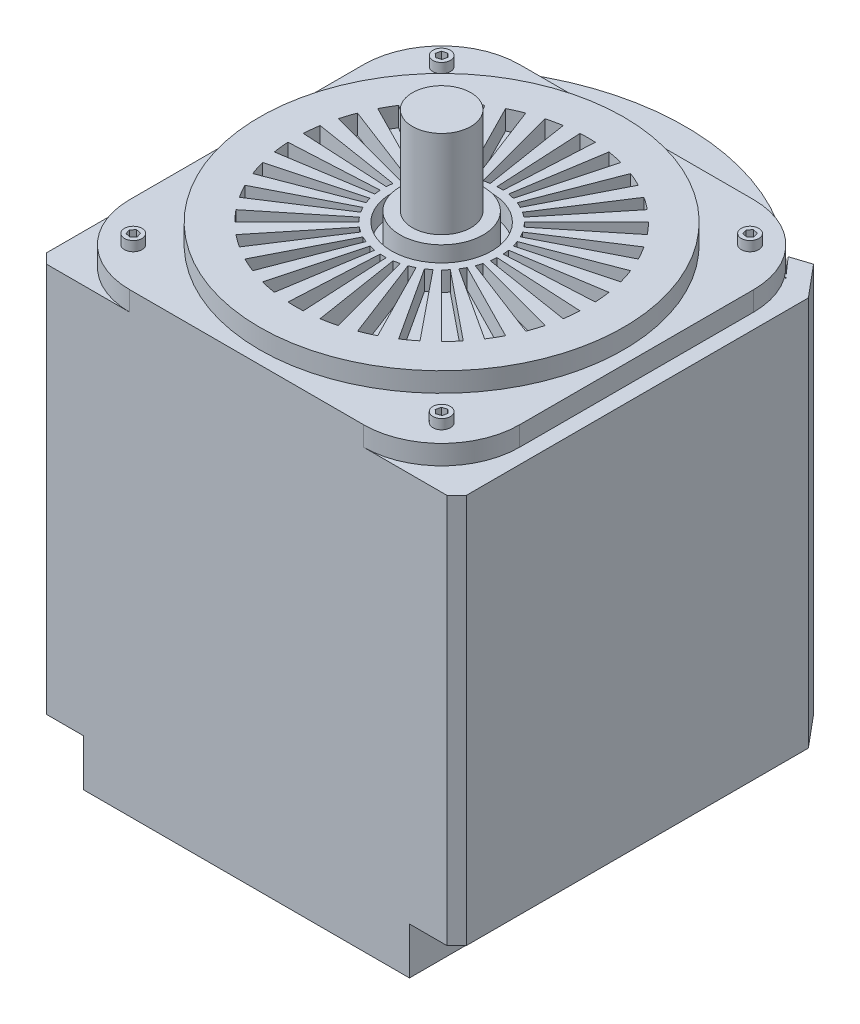
SolidWorks part; units mm, degrees
ref_plane "Front Plane" through (0, 0, 0) normal (0, 0, 1) x (1, 0, 0)
ref_plane "Top Plane" through (0, 0, 0) normal (0, 1, 0) x (1, 0, 0)
ref_plane "Right Plane" through (0, 0, 0) normal (1, 0, 0) x (0, 0, -1)
other "Configuration Table"
sketch "Sketch1" plane through (0, 0, 0) normal (0, 1, 0) x (1, 0, 0)
  line L0 (-1.5, 124.991) -> (-5.5544, 109.8597)
  line L1 (1.5, 124.991) -> (5.5544, 109.8597)
  line L2 (0, 125) -> (0, 0) construction
  line L3 (15.8617, 123.9895) -> (9.7465, 109.5674)
  line L4 (18.8327, 123.5732) -> (20.7479, 108.0256)
  line L5 (32.9165, 120.5882) -> (24.8588, 107.1543)
  line L6 (35.8009, 119.7635) -> (35.5397, 104.1006)
  line L7 (49.3341, 114.8527) -> (39.4899, 102.6672)
  line L8 (52.0761, 113.6357) -> (49.6436, 98.1606)
  line L9 (64.7968, 106.8942) -> (53.3567, 96.1928)
  line L10 (67.3434, 105.3084) -> (62.7867, 90.3207)
  line L11 (79.0053, 96.8667) -> (66.1907, 87.8566)
  line L12 (81.3072, 94.9428) -> (74.7145, 80.7326)
  line L13 (91.6846, 84.9643) -> (77.7436, 77.8199)
  line L15 (0, 0) -> (5.5544, 109.8597) construction
  line L16 (0, 0) -> (20.7479, 108.0256) construction
  line L17 (-15.91, 123.9834) -> (-9.7891, 109.5636)
  line L18 (-18.8808, 123.5658) -> (-20.7899, 108.0175)
  line L19 (-33.0103, 120.5625) -> (-24.9422, 107.1349)
  line L20 (-35.8941, 119.7356) -> (-35.6207, 104.0729)
  line L21 (-49.4681, 114.7951) -> (-39.6097, 102.621)
  line L22 (-52.2087, 113.5749) -> (-49.7582, 98.1026)
  line L23 (-64.9631, 106.7933) -> (-53.5063, 96.1097)
  line L24 (-67.5072, 105.2035) -> (-62.9272, 90.2229)
  line L25 (-79.1936, 96.7128) -> (-66.3615, 87.7277)
  line L26 (-81.4917, 94.7845) -> (-74.8714, 80.5871)
  line L27 (-91.8827, 84.75) -> (-77.925, 77.6382)
  line L29 (0, 0) -> (5.5544, 109.8597) construction
  line L30 (0, 0) -> (-9.7891, 109.5636) construction
  line L31 (93.6972, 82.7395) -> (93.6972, -82.5206)
  line L32 (-93.8901, 82.5206) -> (-93.8901, -82.5206)
  line L33 (-93.8901, -82.5206) -> (93.6972, -82.5206)
  line L35 (-93.8901, 82.5206) -> (-85.3583, 69.3827) [skipped]
  line L36 (93.6972, 82.7395) -> (85.1961, 69.5818) [skipped]
  arc A0 (-91.8827, 84.75) -> (-93.8901, 82.5206) centre (0, 0) ccw
  arc A2 (-79.1936, 96.7128) -> (-81.4917, 94.7845) centre (0, 0) ccw
  arc A3 (-64.9631, 106.7933) -> (-67.5072, 105.2035) centre (0, 0) ccw
  arc A4 (-49.4681, 114.7951) -> (-52.2087, 113.5749) centre (0, 0) ccw
  arc A5 (-33.0103, 120.5625) -> (-35.8941, 119.7356) centre (0, 0) ccw
  arc A6 (-15.91, 123.9834) -> (-18.8808, 123.5658) centre (0, 0) ccw
  arc A7 (1.5, 124.991) -> (-1.5, 124.991) centre (0, 0) ccw
  arc A8 (18.8327, 123.5732) -> (15.8617, 123.9895) centre (0, 0) ccw
  arc A9 (35.8009, 119.7635) -> (32.9165, 120.5882) centre (0, 0) ccw
  arc A10 (52.0761, 113.6357) -> (49.3341, 114.8527) centre (0, 0) ccw
  arc A11 (81.3072, 94.9428) -> (79.0053, 96.8667) centre (0, 0) ccw
  arc A12 (67.3434, 105.3084) -> (64.7968, 106.8942) centre (0, 0) ccw
  arc A13 (-74.8714, 80.5871) -> (-77.925, 77.6382) centre (0, 0) ccw
  arc A14 (-62.9272, 90.2229) -> (-66.3615, 87.7277) centre (0, 0) ccw
  arc A15 (-49.7582, 98.1026) -> (-53.5063, 96.1097) centre (0, 0) ccw
  arc A16 (-35.6207, 104.0729) -> (-39.6097, 102.621) centre (0, 0) ccw
  arc A17 (-20.7899, 108.0175) -> (-24.9422, 107.1349) centre (0, 0) ccw
  arc A18 (-5.5544, 109.8597) -> (-9.7891, 109.5636) centre (0, 0) ccw
  arc A19 (9.7465, 109.5674) -> (5.5544, 109.8597) centre (0, 0) ccw
  arc A20 (24.8588, 107.1543) -> (20.7479, 108.0256) centre (0, 0) ccw
  arc A21 (39.4899, 102.6672) -> (35.5397, 104.1006) centre (0, 0) ccw
  arc A22 (53.3567, 96.1928) -> (49.6436, 98.1606) centre (0, 0) ccw
  arc A23 (66.1907, 87.8566) -> (62.7867, 90.3207) centre (0, 0) ccw
  arc A24 (77.7436, 77.8199) -> (74.7145, 80.7326) centre (0, 0) ccw
  arc A25 (93.6972, 82.7395) -> (91.6846, 84.9643) centre (0, 0) ccw
  point P4 (0, 125)
  dimension "D1" = 250
  dimension "D3" = 1.5
  dimension "D4" = 1.5
  dimension "D5" = 30
  dimension "D6" = 15
  dimension "D8" = 7.978
  dimension "D10" = 8
  dimension "D7" = 7
  dimension "D9" = 7
extrude "Boss-Extrude1" add sketch "Sketch1" along normal blind 200
sketch "Sketch2" plane through (0, 200, 0) normal (0, 1, 0) x (1, 0, 0)
  line L0 (-93.8901, 82.5206) -> (-84.247, 93.4923)
  line L1 (-84.247, 93.4923) -> (-94.0444, 96.7026)
  line L2 (-94.0444, 96.7026) -> (-107.6972, 80.4015)
  line L3 (-107.6972, 80.4015) -> (-107.6972, -82.5206)
  line L4 (-107.6972, -82.5206) -> (-93.8901, -82.5206)
  line L5 (-93.8901, 82.5206) -> (-93.8901, -82.5206)
  line L6 (-93.8901, 82.5206) -> (-93.8901, -82.5206) construction
  line L7 (0, -110) -> (0, 110) construction
  line L8 (93.6972, 82.7395) -> (93.6972, -82.5206)
  line L9 (107.6972, -82.5206) -> (93.6972, -82.5206)
  line L10 (107.6972, 80.4015) -> (107.6972, -82.5206)
  line L11 (94.0444, 96.7026) -> (107.6972, 80.4015)
  line L12 (84.247, 93.4923) -> (94.0444, 96.7026)
  line L13 (93.6972, 82.7395) -> (84.247, 93.4923)
  arc A0 (-91.8827, 84.75) -> (-93.8901, 82.5206) centre (0, 0) ccw construction
  dimension "D1" = 14
  dimension "D2" = 13.8071
extrude "Boss-Extrude2" add sketch "Sketch2" against normal blind 200
sketch "Sketch3" plane through (0, 200, 0) normal (0, 1, 0) x (1, 0, 0)
  line L1 (-60, -100) -> (60, -100)
  line L2 (-100, -60) -> (-100, 60)
  line L3 (-60, 100) -> (60, 100)
  line L4 (100, -60) -> (100, 60)
  line L5 (-88.2843, -88.2843) -> (88.2843, 88.2843) construction
  line L6 (-88.2843, 88.2843) -> (88.2843, -88.2843) construction
  arc A0 (-60, 100) -> (-100, 60) centre (-60, 60) ccw
  arc A1 (100, 60) -> (60, 100) centre (60, 60) ccw
  arc A2 (60, -100) -> (100, -60) centre (60, -60) ccw
  arc A3 (-100, -60) -> (-60, -100) centre (-60, -60) ccw
  point P0 (0, 0)
  dimension "D2" = 40
  dimension "D1" = 4
extrude "Boss-Extrude5" add sketch "Sketch3" along normal blind 10
sketch "Sketch4" plane through (0, 0, 82.5206) normal (0, 0, 1) x (1, 0, 0)
  line L1 (-107.6972, 200) -> (107.6972, 200)
  line L2 (-107.6972, 200) -> (-107.6972, 0)
  line L3 (-107.6972, 0) -> (107.6972, 0)
  line L4 (107.6972, 200) -> (107.6972, 0)
extrude "Boss-Extrude6" add sketch "Sketch4" along normal up to surface (17.4794 mm away) up to face at (0, 205, 100)
sketch "Sketch5" plane through (0, 200, 0) normal (0, 1, 0) x (1, 0, 0)
  line L0 (-102.4593, 71.6037) -> (0, 0)
  line L1 (0, 0) -> (95.1938, 81.0133)
  arc A0 (95.1938, 81.0133) -> (-102.4593, 71.6037) centre (0, 0) ccw
extrude "Boss-Extrude7" add sketch "Sketch5" against normal blind 30
ref_plane "Plane1" through (0, 100, 0) normal (0, -1, 0) x (-1, 0, 0)
mirror "Mirror2" about plane through (0, 100, 0) normal (0, -1, 0) of "Boss-Extrude7"
sketch "Sketch6" plane through (0, 210, 0) normal (0, 1, 0) x (1, 0, 0)
  line L0 (-3.9252, 74.8972) -> (-1.5701, 29.9589)
  line L1 (3.9252, 74.8972) -> (1.5701, 29.9589)
  line L2 (0, -115.5) -> (0, 115.5) construction
  line L3 (11.7326, 74.0766) -> (4.693, 29.6307)
  line L4 (19.4114, 72.4444) -> (7.7646, 28.9778)
  line L5 (26.8776, 70.0185) -> (10.751, 28.0074)
  line L6 (34.0493, 66.8255) -> (13.6197, 26.7302)
  line L7 (40.8479, 62.9003) -> (16.3392, 25.1601)
  line L8 (47.199, 58.2859) -> (18.8796, 23.3144)
  line L9 (53.033, 53.033) -> (21.2132, 21.2132)
  line L10 (58.2859, 47.199) -> (23.3144, 18.8796)
  line L11 (62.9003, 40.8479) -> (25.1601, 16.3392)
  line L12 (66.8255, 34.0493) -> (26.7302, 13.6197)
  line L13 (70.0185, 26.8776) -> (28.0074, 10.751)
  line L14 (72.4444, 19.4114) -> (28.9778, 7.7646)
  line L15 (74.0766, 11.7326) -> (29.6307, 4.693)
  line L16 (74.8972, 3.9252) -> (29.9589, 1.5701)
  line L17 (74.8972, -3.9252) -> (29.9589, -1.5701)
  line L18 (74.0766, -11.7326) -> (29.6307, -4.693)
  line L19 (72.4444, -19.4114) -> (28.9778, -7.7646)
  line L20 (70.0185, -26.8776) -> (28.0074, -10.751)
  line L21 (66.8255, -34.0493) -> (26.7302, -13.6197)
  line L22 (62.9003, -40.8479) -> (25.1601, -16.3392)
  line L23 (58.2859, -47.199) -> (23.3144, -18.8796)
  line L24 (53.033, -53.033) -> (21.2132, -21.2132)
  line L25 (47.199, -58.2859) -> (18.8796, -23.3144)
  line L26 (40.8479, -62.9003) -> (16.3392, -25.1601)
  line L27 (34.0493, -66.8255) -> (13.6197, -26.7302)
  line L28 (26.8776, -70.0185) -> (10.751, -28.0074)
  line L29 (19.4114, -72.4444) -> (7.7646, -28.9778)
  line L30 (11.7326, -74.0766) -> (4.693, -29.6307)
  line L31 (3.9252, -74.8972) -> (1.5701, -29.9589)
  line L32 (-3.9252, -74.8972) -> (-1.5701, -29.9589)
  line L33 (-11.7326, -74.0766) -> (-4.693, -29.6307)
  line L34 (-19.4114, -72.4444) -> (-7.7646, -28.9778)
  line L35 (-26.8776, -70.0185) -> (-10.751, -28.0074)
  line L36 (-34.0493, -66.8255) -> (-13.6197, -26.7302)
  line L37 (-40.8479, -62.9003) -> (-16.3392, -25.1601)
  line L38 (-47.199, -58.2859) -> (-18.8796, -23.3144)
  line L39 (-53.033, -53.033) -> (-21.2132, -21.2132)
  line L40 (-58.2859, -47.199) -> (-23.3144, -18.8796)
  line L41 (-62.9003, -40.8479) -> (-25.1601, -16.3392)
  line L42 (-66.8255, -34.0493) -> (-26.7302, -13.6197)
  line L43 (-70.0185, -26.8776) -> (-28.0074, -10.751)
  line L44 (-72.4444, -19.4114) -> (-28.9778, -7.7646)
  line L45 (-74.0766, -11.7326) -> (-29.6307, -4.693)
  line L46 (-74.8972, -3.9252) -> (-29.9589, -1.5701)
  line L47 (-74.8972, 3.9252) -> (-29.9589, 1.5701)
  line L48 (-74.0766, 11.7326) -> (-29.6307, 4.693)
  line L49 (-72.4444, 19.4114) -> (-28.9778, 7.7646)
  line L50 (-70.0185, 26.8776) -> (-28.0074, 10.751)
  line L51 (-66.8255, 34.0493) -> (-26.7302, 13.6197)
  line L52 (-62.9003, 40.8479) -> (-25.1601, 16.3392)
  line L53 (-58.2859, 47.199) -> (-23.3144, 18.8796)
  line L54 (-53.033, 53.033) -> (-21.2132, 21.2132)
  line L55 (-47.199, 58.2859) -> (-18.8796, 23.3144)
  line L56 (-40.8479, 62.9003) -> (-16.3392, 25.1601)
  line L57 (-34.0493, 66.8255) -> (-13.6197, 26.7302)
  line L58 (-26.8776, 70.0185) -> (-10.751, 28.0074)
  line L59 (-19.4114, 72.4444) -> (-7.7646, 28.9778)
  line L60 (-11.7326, 74.0766) -> (-4.693, 29.6307)
  circle A0 centre (0, 0) radius 93.3948
  arc A1 (3.9252, 74.8972) -> (-3.9252, 74.8972) centre (0, 0) ccw
  arc A2 (1.5701, 29.9589) -> (-1.5701, 29.9589) centre (0, 0) ccw
  arc A3 (7.7646, 28.9778) -> (4.693, 29.6307) centre (0, 0) ccw
  arc A4 (19.4114, 72.4444) -> (11.7326, 74.0766) centre (0, 0) ccw
  arc A5 (13.6197, 26.7302) -> (10.751, 28.0074) centre (0, 0) ccw
  arc A6 (34.0493, 66.8255) -> (26.8776, 70.0185) centre (0, 0) ccw
  arc A7 (18.8796, 23.3144) -> (16.3392, 25.1601) centre (0, 0) ccw
  arc A8 (47.199, 58.2859) -> (40.8479, 62.9003) centre (0, 0) ccw
  arc A9 (23.3144, 18.8796) -> (21.2132, 21.2132) centre (0, 0) ccw
  arc A10 (58.2859, 47.199) -> (53.033, 53.033) centre (0, 0) ccw
  arc A11 (26.7302, 13.6197) -> (25.1601, 16.3392) centre (0, 0) ccw
  arc A12 (66.8255, 34.0493) -> (62.9003, 40.8479) centre (0, 0) ccw
  arc A13 (28.9778, 7.7646) -> (28.0074, 10.751) centre (0, 0) ccw
  arc A14 (72.4444, 19.4114) -> (70.0185, 26.8776) centre (0, 0) ccw
  arc A15 (29.9589, 1.5701) -> (29.6307, 4.693) centre (0, 0) ccw
  arc A16 (74.8972, 3.9252) -> (74.0766, 11.7326) centre (0, 0) ccw
  arc A17 (29.6307, -4.693) -> (29.9589, -1.5701) centre (0, 0) ccw
  arc A18 (74.0766, -11.7326) -> (74.8972, -3.9252) centre (0, 0) ccw
  arc A19 (28.0074, -10.751) -> (28.9778, -7.7646) centre (0, 0) ccw
  arc A20 (70.0185, -26.8776) -> (72.4444, -19.4114) centre (0, 0) ccw
  arc A21 (25.1601, -16.3392) -> (26.7302, -13.6197) centre (0, 0) ccw
  arc A22 (62.9003, -40.8479) -> (66.8255, -34.0493) centre (0, 0) ccw
  arc A23 (21.2132, -21.2132) -> (23.3144, -18.8796) centre (0, 0) ccw
  arc A24 (53.033, -53.033) -> (58.2859, -47.199) centre (0, 0) ccw
  arc A25 (16.3392, -25.1601) -> (18.8796, -23.3144) centre (0, 0) ccw
  arc A26 (40.8479, -62.9003) -> (47.199, -58.2859) centre (0, 0) ccw
  arc A27 (10.751, -28.0074) -> (13.6197, -26.7302) centre (0, 0) ccw
  arc A28 (26.8776, -70.0185) -> (34.0493, -66.8255) centre (0, 0) ccw
  arc A29 (4.693, -29.6307) -> (7.7646, -28.9778) centre (0, 0) ccw
  arc A30 (11.7326, -74.0766) -> (19.4114, -72.4444) centre (0, 0) ccw
  arc A31 (-1.5701, -29.9589) -> (1.5701, -29.9589) centre (0, 0) ccw
  arc A32 (-3.9252, -74.8972) -> (3.9252, -74.8972) centre (0, 0) ccw
  arc A33 (-7.7646, -28.9778) -> (-4.693, -29.6307) centre (0, 0) ccw
  arc A34 (-19.4114, -72.4444) -> (-11.7326, -74.0766) centre (0, 0) ccw
  arc A35 (-13.6197, -26.7302) -> (-10.751, -28.0074) centre (0, 0) ccw
  arc A36 (-34.0493, -66.8255) -> (-26.8776, -70.0185) centre (0, 0) ccw
  arc A37 (-18.8796, -23.3144) -> (-16.3392, -25.1601) centre (0, 0) ccw
  arc A38 (-47.199, -58.2859) -> (-40.8479, -62.9003) centre (0, 0) ccw
  arc A39 (-23.3144, -18.8796) -> (-21.2132, -21.2132) centre (0, 0) ccw
  arc A40 (-58.2859, -47.199) -> (-53.033, -53.033) centre (0, 0) ccw
  arc A41 (-26.7302, -13.6197) -> (-25.1601, -16.3392) centre (0, 0) ccw
  arc A42 (-66.8255, -34.0493) -> (-62.9003, -40.8479) centre (0, 0) ccw
  arc A43 (-28.9778, -7.7646) -> (-28.0074, -10.751) centre (0, 0) ccw
  arc A44 (-72.4444, -19.4114) -> (-70.0185, -26.8776) centre (0, 0) ccw
  arc A45 (-29.9589, -1.5701) -> (-29.6307, -4.693) centre (0, 0) ccw
  arc A46 (-74.8972, -3.9252) -> (-74.0766, -11.7326) centre (0, 0) ccw
  arc A47 (-29.6307, 4.693) -> (-29.9589, 1.5701) centre (0, 0) ccw
  arc A48 (-74.0766, 11.7326) -> (-74.8972, 3.9252) centre (0, 0) ccw
  arc A49 (-28.0074, 10.751) -> (-28.9778, 7.7646) centre (0, 0) ccw
  arc A50 (-70.0185, 26.8776) -> (-72.4444, 19.4114) centre (0, 0) ccw
  arc A51 (-25.1601, 16.3392) -> (-26.7302, 13.6197) centre (0, 0) ccw
  arc A52 (-62.9003, 40.8479) -> (-66.8255, 34.0493) centre (0, 0) ccw
  arc A53 (-21.2132, 21.2132) -> (-23.3144, 18.8796) centre (0, 0) ccw
  arc A54 (-53.033, 53.033) -> (-58.2859, 47.199) centre (0, 0) ccw
  arc A55 (-16.3392, 25.1601) -> (-18.8796, 23.3144) centre (0, 0) ccw
  arc A56 (-40.8479, 62.9003) -> (-47.199, 58.2859) centre (0, 0) ccw
  arc A57 (-10.751, 28.0074) -> (-13.6197, 26.7302) centre (0, 0) ccw
  arc A58 (-26.8776, 70.0185) -> (-34.0493, 66.8255) centre (0, 0) ccw
  arc A59 (-4.693, 29.6307) -> (-7.7646, 28.9778) centre (0, 0) ccw
  arc A60 (-11.7326, 74.0766) -> (-19.4114, 72.4444) centre (0, 0) ccw
  circle A61 centre (0, 0) radius 25.6738
  dimension "D3" = 75
  dimension "D4" = 30
  dimension "D1" = 3
  dimension "D2" = 3
  dimension "D5" = 30
extrude "Boss-Extrude8" add sketch "Sketch6" along normal blind 10
sketch "Sketch7" plane through (0, 210, 0) normal (0, 1, 0) x (1, 0, 0)
  circle A0 centre (0, 0) radius 21.3319
extrude "Boss-Extrude9" add sketch "Sketch7" along normal blind 15
sketch "Sketch8" plane through (0, 225, 0) normal (0, 1, 0) x (1, 0, 0)
  circle A0 centre (0, 0) radius 15
  dimension "D1" = 30
extrude "Boss-Extrude10" add sketch "Sketch8" along normal blind 45
sketch "Sketch9" plane through (0, 210, 0) normal (0, 1, 0) x (1, 0, 0)
  line L0 (-88.2843, 88.2843) -> (0, 0) construction
  arc A0 (-60, 100) -> (-100, 60) centre (-60, 60) ccw construction
  circle A1 centre (-79.0919, 79.0919) radius 4.5
  point P0 (-88.2843, 88.2843)
  dimension "D1" = 9
  dimension "D2" = 13
extrude "Boss-Extrude11" add sketch "Sketch9" along normal blind 5
sketch "Sketch10" plane through (0, 215, 0) normal (0, 1, 0) x (1, 0, 0)
  line L1 (-77.137, 77.3381) -> (-76.5956, 79.908)
  line L2 (-76.5956, 79.908) -> (-78.5505, 81.6618)
  line L3 (-78.5505, 81.6618) -> (-81.0468, 80.8457)
  line L4 (-81.0468, 80.8457) -> (-81.5882, 78.2758)
  line L5 (-81.5882, 78.2758) -> (-79.6333, 76.522)
  line L6 (-79.6333, 76.522) -> (-77.137, 77.3381)
  circle A0 centre (-79.0919, 79.0919) radius 2.2744 construction
extrude "Cut-Extrude1" cut sketch "Sketch10" against normal blind 4
pattern_circular "CirPattern1" count 4 over 360 about axis through (0, 0, 0) along (0, 1, 0) of "Cut-Extrude1", "Boss-Extrude11"
sketch "Sketch11" plane through (0, 0, 0) normal (0, -1, 0) x (1, 0, 0)
  line L0 (-84.247, -93.4923) -> (-80.9734, -90.2187)
  line L1 (-80.9734, -90.2187) -> (-95.934, -80.8502)
  line L2 (-95.934, -80.8502) -> (-84.247, -93.4923)
  line L3 (84.247, -93.4923) -> (80.6415, -91.2344)
  line L4 (80.6415, -91.2344) -> (99.0626, -78.2916)
  line L5 (99.0626, -78.2916) -> (84.247, -93.4923)
extrude "Boss-Extrude12" add sketch "Sketch11" against normal blind 4
sketch "Sketch12" plane through (0, 0, 0) normal (0, -1, 0) x (1, 0, 0)
  line L0 (-83.6448, -92.89) -> (-83.6448, 100)
  line L1 (107.6972, 100) -> (-107.6972, 100) construction
  line L2 (-83.6448, 100) -> (83.4972, 100)
  line L3 (83.4972, 100) -> (83.4972, -93.0227)
  arc A0 (-83.6448, -92.89) -> (83.4972, -93.0227) centre (0, 0) ccw
extrude "Boss-Extrude13" add sketch "Sketch12" along normal blind 24
chamfer "Chamfer1" distance 5 angle 45 2 edges at (-107.6972, 100, 100) (107.6972, 100, 100)
ref_plane "Plane2" through (0, 0, -125) normal (0, 0, -1) x (-1, 0, 0)
sketch "Sketch13" plane through (0, 0, -125) normal (0, 0, -1) x (-1, 0, 0)
  line L0 (60, 200) -> (-60, 200) construction
  line L1 (-68.4972, 185) -> (68.6448, 185) construction
  line L2 (-68.4972, 185) -> (-68.4972, -9) construction
  line L3 (-68.4972, -9) -> (68.6448, -9) construction
  line L4 (68.6448, 185) -> (68.6448, -9) construction
  line L5 (-83.4972, -24) -> (-83.4972, 0) construction
  line L6 (83.6448, -24) -> (83.6448, 0) construction
  line L7 (-83.4972, -24) -> (83.6448, -24) construction
  circle A0 centre (-68.4972, 185) radius 6.5
  circle A1 centre (68.6448, 185) radius 6.5
  circle A2 centre (-68.4972, -9) radius 6.5
  circle A3 centre (68.6448, -9) radius 6.5
  dimension "D5" = 13
  dimension "D1" = 15
  dimension "D2" = 15
  dimension "D3" = 15
  dimension "D4" = 15
extrude "Cut-Extrude2" cut sketch "Sketch13" against normal blind 30
sketch "Sketch14" plane through (0, 0, -95) normal (0, 0, -1) x (-1, 0, 0)
  line L1 (-65.7113, 183.1288) -> (-65.4837, 186.4771)
  line L2 (-65.4837, 186.4771) -> (-68.2696, 188.3482)
  line L3 (-68.2696, 188.3482) -> (-71.2831, 186.8712)
  line L4 (-71.2831, 186.8712) -> (-71.5106, 183.5229)
  line L5 (-71.5106, 183.5229) -> (-68.7247, 181.6518)
  line L6 (-68.7247, 181.6518) -> (-65.7113, 183.1288)
  line L7 (69.7434, 181.6518) -> (72.0937, 184.2773)
  line L8 (72.0937, 184.2773) -> (70.9951, 187.6256)
  line L9 (70.9951, 187.6256) -> (67.5461, 188.3482)
  line L10 (67.5461, 188.3482) -> (65.1958, 185.7227)
  line L11 (65.1958, 185.7227) -> (66.2944, 182.3744)
  line L12 (66.2944, 182.3744) -> (69.7434, 181.6518)
  line L13 (70.8936, -11.049) -> (71.5436, -8.0769)
  line L14 (71.5436, -8.0769) -> (69.2948, -6.0279)
  line L15 (69.2948, -6.0279) -> (66.3959, -6.951)
  line L16 (66.3959, -6.951) -> (65.7459, -9.9231)
  line L17 (65.7459, -9.9231) -> (67.9947, -11.9721)
  line L18 (67.9947, -11.9721) -> (70.8936, -11.049)
  line L19 (-71.6891, -9.4155) -> (-69.7332, -11.9721)
  line L20 (-69.7332, -11.9721) -> (-66.5413, -11.5565)
  line L21 (-66.5413, -11.5565) -> (-65.3052, -8.5845)
  line L22 (-65.3052, -8.5845) -> (-67.2611, -6.0279)
  line L23 (-67.2611, -6.0279) -> (-70.453, -6.4435)
  line L24 (-70.453, -6.4435) -> (-71.6891, -9.4155)
  circle A0 centre (-68.4972, 185) radius 5.5
  circle A1 centre (-68.4972, 185) radius 2.9064 construction
  circle A2 centre (68.6448, 185) radius 5.5
  circle A3 centre (-68.4972, -9) radius 5.5
  circle A4 centre (68.6448, -9) radius 5.5
  circle A5 centre (68.6448, 185) radius 3.0518 construction
  circle A6 centre (68.6448, -9) radius 2.6347 construction
  circle A7 centre (-68.4972, -9) radius 2.7876 construction
  dimension "D1" = 11
  dimension "D2" = 11
extrude "Boss-Extrude14" add sketch "Sketch14" along normal blind 4
